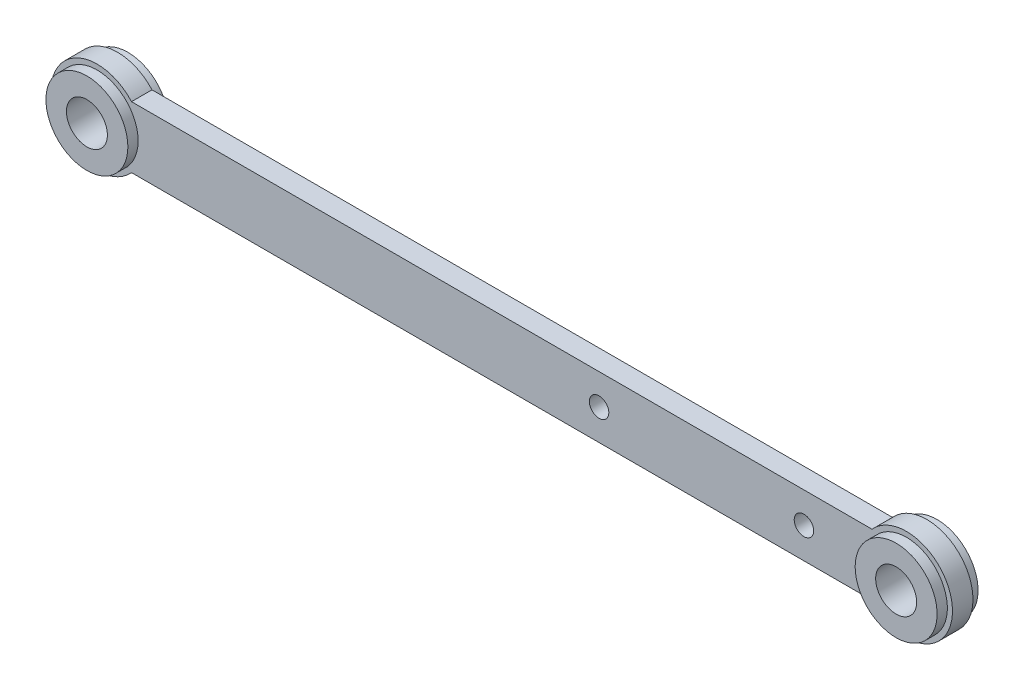
from build123d import *

# Parameters (mm, degrees)
SKETCH_1_R          = 20
EXTRUDE_1_DEPTH     = 20
SKETCH_2_R          = 40
SKETCH_2_R_2        = 20
EXTRUDE_2_DEPTH     = 10
EXTRUDE_START       = 10
SKETCH_3_R          = 40
SKETCH_3_R_2        = 20
EXTRUDE_3_DEPTH     = 10
HOLE_WIZARD_M16_1_D = 19


with BuildPart() as part:
    # 草图1 → 凸台-拉伸1 (new body)
    with BuildSketch(Plane.XY):
        with BuildLine():
            ThreePointArc((361.458980338, -30), (440, 0), (361.458980338, 30))
            Line((361.458980338, 30), (-361.458980338, 30))
            ThreePointArc((-361.458980338, 30), (-440, 0), (-361.458980338, -30))
            Line((-361.458980338, -30), (361.458980338, -30))
        make_face()
        with Locations((395, 0)):
            Circle(SKETCH_1_R, mode=Mode.SUBTRACT)
        with Locations((-395, 0)):
            Circle(SKETCH_1_R, mode=Mode.SUBTRACT)
    extrude(amount=EXTRUDE_1_DEPTH)

    # 草图2 → 凸台-拉伸2 (add)
    # profile 1 of 2: a face of its own
    with BuildSketch(Plane.XY.offset(20)):
        with Locations((-395, 0)):
            Circle(SKETCH_2_R)
        with Locations((-395, 0)):
            Circle(SKETCH_2_R_2, mode=Mode.SUBTRACT)
    # profile 2 of 2: a face of its own
    with BuildSketch(Plane.XY.offset(20)):
        with Locations(Location((395, 0, 0), (0, 0, 180))):
            Circle(SKETCH_2_R)
        with Locations(Location((395, 0, 0), (0, 0, 180))):
            Circle(SKETCH_2_R_2, mode=Mode.SUBTRACT)
    extrude(amount=EXTRUDE_2_DEPTH)

    # 草图3 → 凸台-拉伸3 (add)
    # profile 1 of 2: a face of its own
    with BuildSketch(Plane(origin=(0, 0, 0), x_dir=(-1, 0, 0), z_dir=(0, 0, -1)).offset(EXTRUDE_START)):
        with Locations((-395, 0)):
            Circle(SKETCH_3_R)
        with Locations((-395, 0)):
            Circle(SKETCH_3_R_2, mode=Mode.SUBTRACT)
    # profile 2 of 2: a face of its own
    with BuildSketch(Plane(origin=(0, 0, 0), x_dir=(-1, 0, 0), z_dir=(0, 0, -1)).offset(EXTRUDE_START)):
        with Locations(Location((395, 0, 0), (0, 0, 180))):
            Circle(SKETCH_3_R)
        with Locations((395, 0)):
            Circle(SKETCH_3_R_2, mode=Mode.SUBTRACT)
    extrude(amount=-EXTRUDE_3_DEPTH)

    # M16 间隙孔1 (through all)
    with Locations(Plane.XY.offset(20)):
        with Locations((95, 0), (295, 0)):
            Hole(HOLE_WIZARD_M16_1_D / 2)


solid = part.part
